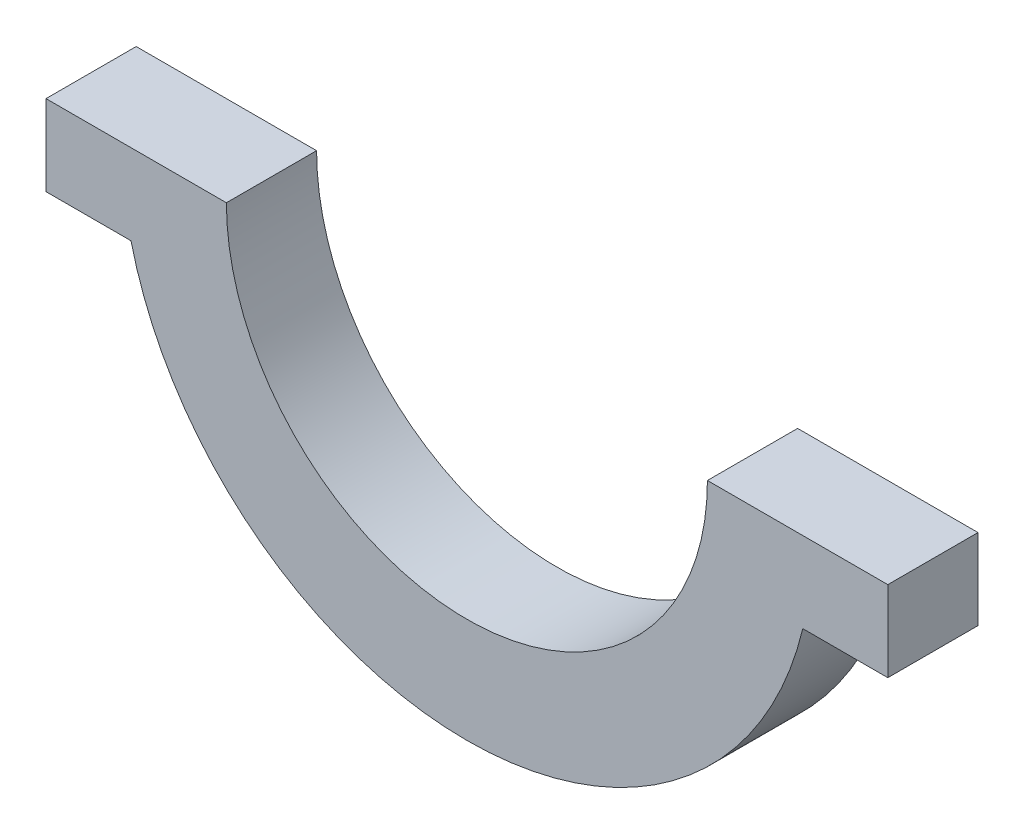
from build123d import *

# Parameters (mm, degrees)
BOSS_EXTRUDE1_DEPTH = 6


with BuildPart() as part:
    # Sketch1 → Boss-Extrude1 (new body)
    with BuildSketch(Plane.XY):
        with BuildLine():
            Line((-16, 50), (-28, 50))
            Line((-28, 50), (-28, 44.637095603))
            Line((-28, 44.637095603), (-22.344508596, 44.637095603))
            ThreePointArc((-22.344508596, 44.637095603), (0, 27.020926738), (22.344508596, 44.637095603))
            Line((22.344508596, 44.637095603), (28, 44.637095603))
            Line((28, 44.637095603), (28, 50))
            Line((28, 50), (16, 50))
            ThreePointArc((16, 50), (0, 34), (-16, 50))
        make_face()
    extrude(amount=BOSS_EXTRUDE1_DEPTH)


solid = part.part
